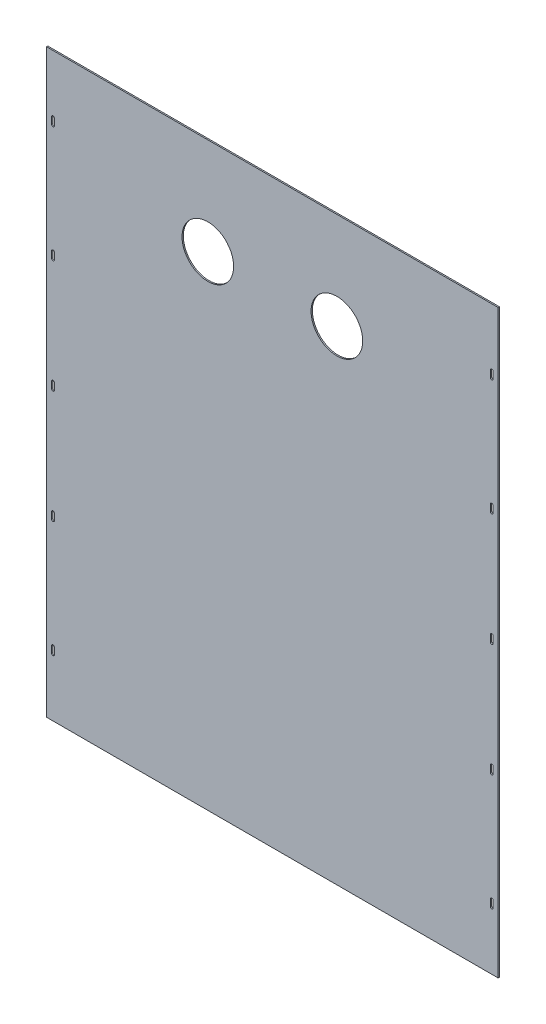
SolidWorks part; units mm, degrees
material "Q235A"
ref_plane "前视基准面" through (0, 0, 0) normal (0, 0, 1) x (1, 0, 0)
ref_plane "上视基准面" through (0, 0, 0) normal (0, 1, 0) x (1, 0, 0)
ref_plane "右视基准面" through (0, 0, 0) normal (1, 0, 0) x (0, 0, -1)
sketch "草图1" plane through (0, 0, 0) normal (0, 0, 1) x (1, 0, 0)
  line L1 (-350, 450) -> (350, 450)
  line L2 (-350, 450) -> (-350, -450)
  line L3 (-350, -450) -> (350, -450)
  line L4 (350, 450) -> (350, -450)
  line L5 (0, -450) -> (0, 450) construction
  line L6 (-350, 0) -> (350, 0) construction
  point P0 (0, 0)
  dimension "D1" = 700
  dimension "D2" = 900
extrude "凸台-拉伸1" add sketch "草图1" along normal blind 2
sketch "草图2" plane through (0, 0, 2) normal (0, 0, 1) x (1, 0, 0)
  line L0 (0, 450) -> (0, -450) construction
  line L1 (350, 450) -> (-350, 450) construction
  line L2 (-350, -450) -> (350, -450) construction
  line L3 (-340, 180) -> (-340, 170) construction
  line L4 (-340, -175) -> (340, -175) construction
  line L5 (-340, -175) -> (-340, 175) construction
  line L6 (-340, 175) -> (340, 175) construction
  line L7 (340, -175) -> (340, 175) construction
  line L8 (0, 175) -> (0, -175) construction
  line L9 (-340, 0) -> (340, 0) construction
  line L10 (-337.75, 180) -> (-337.75, 170)
  line L11 (-342.25, 180) -> (-342.25, 170)
  line L12 (340, 170) -> (340, 180) construction
  line L15 (340, 360) -> (340, 350) construction
  line L18 (-340, -5) -> (-340, 5) construction
  line L19 (-342.25, -5) -> (-342.25, 5)
  line L20 (-337.75, -5) -> (-337.75, 5)
  line L21 (337.75, 170) -> (337.75, 180)
  line L24 (340, -5) -> (340, 5) construction
  line L25 (342.25, -5) -> (342.25, 5)
  line L26 (337.75, -5) -> (337.75, 5)
  line L27 (-340, 360) -> (-340, 350) construction
  line L28 (-342.25, 360) -> (-342.25, 350)
  line L29 (-337.75, 360) -> (-337.75, 350)
  line L30 (342.25, 170) -> (342.25, 180)
  line L33 (-340, -175) -> (340, -175) construction
  line L34 (340, -170) -> (340, -180) construction
  line L37 (337.75, -170) -> (337.75, -180)
  line L40 (342.25, -170) -> (342.25, -180)
  line L43 (-340, -170) -> (-340, -180) construction
  line L46 (340, -355) -> (-340, -355) construction
  line L47 (340, -355) -> (340, 355) construction
  line L48 (340, 355) -> (-340, 355) construction
  line L49 (-340, -355) -> (-340, 355) construction
  line L50 (0, 355) -> (0, -355) construction
  line L51 (340, 0) -> (-340, 0) construction
  line L52 (342.25, 360) -> (342.25, 350)
  line L53 (337.75, 360) -> (337.75, 350)
  line L54 (340, -355) -> (-340, -355) construction
  line L55 (340, -360) -> (340, -350) construction
  line L56 (342.25, -360) -> (342.25, -350)
  line L57 (337.75, -360) -> (337.75, -350)
  line L58 (-340, -360) -> (-340, -350) construction
  line L59 (-342.25, -360) -> (-342.25, -350)
  line L60 (-337.75, -360) -> (-337.75, -350)
  line L61 (-337.75, -170) -> (-337.75, -180)
  line L62 (-342.25, -170) -> (-342.25, -180)
  arc A0 (-337.75, 180) -> (-342.25, 180) centre (-340, 180) ccw
  arc A1 (-342.25, 170) -> (-337.75, 170) centre (-340, 170) ccw
  arc A6 (-342.25, -5) -> (-337.75, -5) centre (-340, -5) ccw
  arc A7 (-337.75, 5) -> (-342.25, 5) centre (-340, 5) ccw
  arc A10 (342.25, -5) -> (337.75, -5) centre (340, -5) cw
  arc A11 (337.75, 5) -> (342.25, 5) centre (340, 5) cw
  arc A12 (-342.25, 360) -> (-337.75, 360) centre (-340, 360) cw
  arc A13 (-337.75, 350) -> (-342.25, 350) centre (-340, 350) cw
  arc A24 (342.25, 360) -> (337.75, 360) centre (340, 360) ccw
  arc A25 (337.75, 350) -> (342.25, 350) centre (340, 350) ccw
  arc A26 (342.25, -360) -> (337.75, -360) centre (340, -360) cw
  arc A27 (337.75, -350) -> (342.25, -350) centre (340, -350) cw
  arc A28 (-342.25, -360) -> (-337.75, -360) centre (-340, -360) ccw
  arc A29 (-337.75, -350) -> (-342.25, -350) centre (-340, -350) ccw
  arc A30 (337.75, 170) -> (342.25, 170) centre (340, 170) ccw
  arc A31 (342.25, 180) -> (337.75, 180) centre (340, 180) ccw
  arc A32 (337.75, -170) -> (342.25, -170) centre (340, -170) cw
  arc A33 (342.25, -180) -> (337.75, -180) centre (340, -180) cw
  arc A34 (-337.75, -170) -> (-342.25, -170) centre (-340, -170) ccw
  arc A35 (-342.25, -180) -> (-337.75, -180) centre (-340, -180) ccw
  point P6 (0, 0)
  point P12 (-340, 175)
  point P18 (340, 175)
  point P24 (0, 0)
  point P32 (-340, 0)
  point P38 (340, -175)
  point P47 (340, 0)
  point P54 (-340, 355)
  point P59 (-340, -175)
  point P95 (340, 355)
  point P102 (340, -355)
  point P109 (-340, -355)
  dimension "D1" = 680
  dimension "D2" = 710
  dimension "D3" = 4.5
  dimension "D4" = 10
  dimension "D5" = 175
  dimension "D6" = 10
  dimension "D7" = 4.5
  dimension "D8" = 4.5
  dimension "D9" = 10
  dimension "D10" = 10
  dimension "D11" = 4.5
extrude "切除-拉伸1" cut sketch "草图2" against normal blind 10
sketch "草图3" plane through (0, 0, 2) normal (0, 0, 1) x (1, 0, 0)
  line L0 (0, 450) -> (0, -450) construction
  line L1 (350, 450) -> (-350, 450) construction
  line L2 (-350, -450) -> (350, -450) construction
  line L3 (-100, 300) -> (100, 300) construction
  circle A0 centre (-100, 300) radius 40
  circle A1 centre (100, 300) radius 40
  dimension "D3" = 80
  dimension "D1" = 150
  dimension "D2" = 200
extrude "切除-拉伸2" cut sketch "草图3" against normal blind 10
